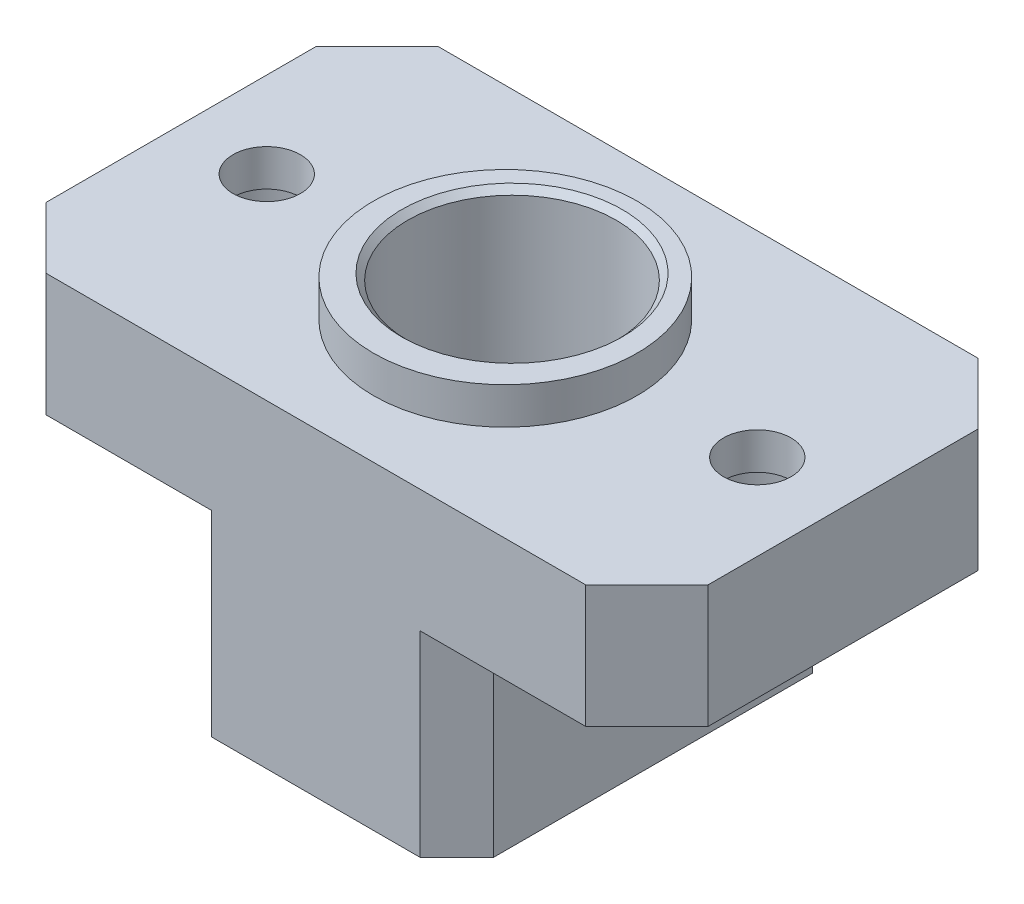
SolidWorks part; units mm, degrees
material "Q235-A"
ref_plane "Front Plane" through (0, 0, 0) normal (0, 0, 1) x (1, 0, 0)
ref_plane "Top Plane" through (0, 0, 0) normal (0, 1, 0) x (1, 0, 0)
ref_plane "Right Plane" through (0, 0, 0) normal (1, 0, 0) x (0, 0, -1)
sketch "Sketch1" plane through (0, 0, 0) normal (0, 0, 1) x (1, 0, 0)
  line L0 (0, 11.4789) -> (0, -20.5384) construction
  line L1 (11.5, -16.0086) -> (-11.5, -16.0086)
  line L2 (-11.5, -16.0086) -> (-11.5, -0.0086)
  line L3 (-11.5, -0.0086) -> (-27, -0.0086)
  line L4 (-27, -0.0086) -> (-27, 9.9914)
  line L5 (-27, 9.9914) -> (27, 9.9914)
  line L6 (11.5, -16.0086) -> (11.5, -0.0086)
  line L7 (11.5, -0.0086) -> (27, -0.0086)
  line L8 (27, -0.0086) -> (27, 9.9914)
  point P10 (0, -16.0086)
  point P13 (0, 9.9914)
  dimension "D1" = 11.5
  dimension "D2" = 10
  dimension "D3" = 16
  dimension "D4" = 15.5
extrude "Boss-Extrude1" add sketch "Sketch1" along normal blind 32
chamfer "Chamfer1" distance 5 angle 45 4 edges at (27, 4.9914, 32) (27, 4.9914, 0) (-27, 4.9914, 32) (-27, 4.9914, 0)
sketch "Sketch2" plane through (0, 9.9914, 0) normal (0, 1, 0) x (1, 0, 0)
  circle A0 centre (0, -16.5471) radius 10.75
extrude "Boss-Extrude2" add sketch "Sketch2" along normal blind 3
sketch "Sketch5" plane through (0, -0.0086, 0) normal (0, -1, 0) x (1, 0, 0)
  line L0 (20, 16) -> (-20, 16)
  line L1 (27, 27) -> (27, 5) construction
  dimension "D1" = 40
  dimension "D2" = 7
hole_wizard "Hole2" positions "Sketch6" profile "Sketch7" legacy
sketch "Sketch6" plane through (0, -0.0086, 0) normal (0, -1, 0) x (-1, 0, 0)
  point P0 (-20, -16)
  point P3 (20, -16)
sketch "Sketch7" plane through (20, -0.0086, 16) normal (1, 0, 0) x (0, 0, -1)
  line L0 (0, 0) -> (0, 100)
  line L1 (0, 100) -> (2.75, 100)
  line L2 (2.75, 100) -> (2.75, 7)
  line L3 (2.75, 7) -> (5, 7)
  line L4 (5, 7) -> (5, 0)
  line L5 (5, 0) -> (0, 0)
  line L6 (0, 110) -> (0, -10) construction
  dimension "直径" = 5.5
  dimension "深度" = 100
  dimension "柱坑直径" = 10
  dimension "柱坑深度" = 7
chamfer "Chamfer3" distance 3 angle 45 4 edges at (-11.5, -8.0086, 32) (-11.5, -8.0086, 0) (11.5, -8.0086, 32) (11.5, -8.0086, 0)
sketch "Sketch9" plane through (0, -16.0086, 0) normal (0, -1, 0) x (1, 0, 0)
  line L0 (0, 0) -> (0, 32)
  line L1 (-8.5, 32) -> (8.5, 32) construction
hole_wizard "Hole3" positions "Sketch10" profile "Sketch11" legacy end condition through all
sketch "Sketch10" plane through (0, -16.0086, 0) normal (0, -1, 0) x (-1, 0, 0)
  line L0 (0, 0) -> (0, -32) construction
  point P0 (0, -16)
sketch "Sketch11" plane through (0, -16.0086, 16) normal (1, 0, 0) x (0, 0, -1)
  line L0 (0, 0) -> (0, 29)
  line L1 (0, 29) -> (8.5, 29)
  line L2 (8.5, 29) -> (8.5, 0)
  line L3 (8.5, 0) -> (0, 0)
  line L4 (0, 110) -> (0, -10) construction
  dimension "直径" = 17
  dimension "深度" = 29
chamfer "Chamfer5" distance 0.5 angle 45 1 edges at (0, 12.9914, 7.5)
chamfer "Chamfer6" distance 1 angle 45 1 edges at (0, -16.0086, 7.5)
